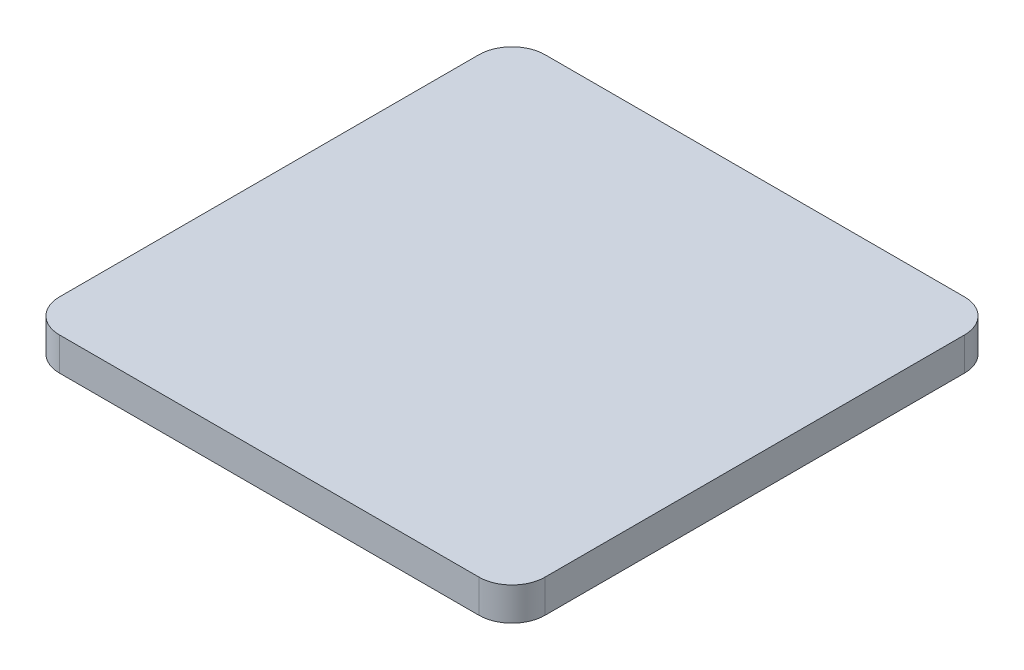
SolidWorks part; units mm, degrees
ref_plane "前视基准面" through (0, 0, 0) normal (0, 0, 1) x (1, 0, 0)
ref_plane "上视基准面" through (0, 0, 0) normal (0, 1, 0) x (1, 0, 0)
ref_plane "右视基准面" through (0, 0, 0) normal (1, 0, 0) x (0, 0, -1)
sketch "草图1" plane through (0, 0, 0) normal (0, 1, 0) x (1, 0, 0)
  line L1 (-22, 22) -> (22, 22)
  line L2 (-22, 22) -> (-22, -22)
  line L3 (-22, -22) -> (22, -22)
  line L4 (22, 22) -> (22, -22)
  line L5 (-22, 22) -> (22, -22) construction
  line L6 (-22, -22) -> (22, 22) construction
  point P0 (0, 0)
  dimension "D1" = 44
  dimension "D2" = 44
extrude "凸台-拉伸1" add sketch "草图1" along normal blind 3
fillet "圆角1" radius 3 4 edges at (-22, 1.5, -22) (22, 1.5, -22) (22, 1.5, 22) (-22, 1.5, 22)
